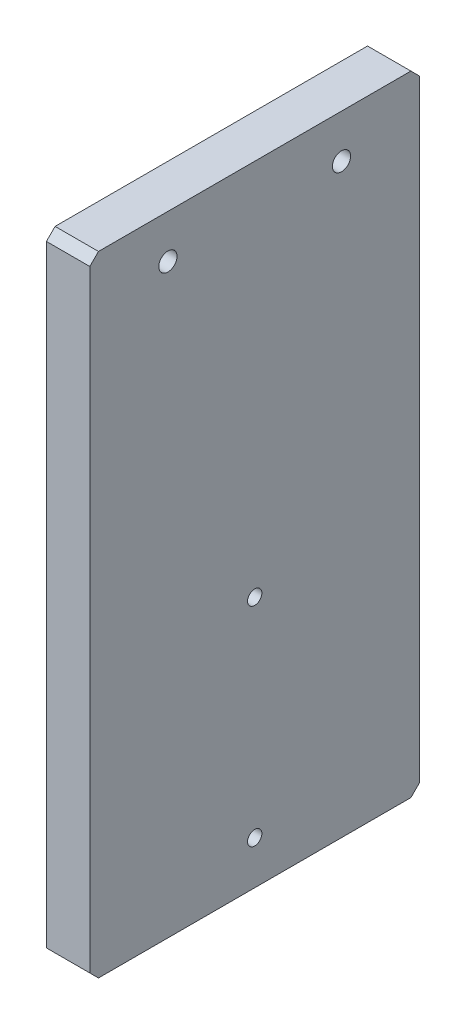
SolidWorks part; units mm, degrees
material "A6061"
ref_plane "前基準面" through (0, 0, 0) normal (0, 0, 1) x (1, 0, 0)
ref_plane "上基準面" through (0, 0, 0) normal (0, 1, 0) x (1, 0, 0)
ref_plane "右基準面" through (0, 0, 0) normal (1, 0, 0) x (0, 0, -1)
sketch "草图1" plane through (0, 0, 0) normal (1, 0, 0) x (0, 0, -1)
  line L1 (-38, 72.5) -> (38, 72.5)
  line L2 (-38, 72.5) -> (-38, -72.5)
  line L3 (-38, -72.5) -> (38, -72.5)
  line L4 (38, 72.5) -> (38, -72.5)
  line L5 (-38, 72.5) -> (38, -72.5) construction
  line L6 (-38, -72.5) -> (38, 72.5) construction
  point P0 (0, 0)
  dimension "D1" = 145
  dimension "D2" = 76
extrude "凸台-拉伸1" add sketch "草图1" along normal blind 10
sketch "草图2" plane through (10, 0, 0) normal (1, 0, 0) x (0, 0, -1)
  line L1 (38, 72.5) -> (-38, 72.5)
  line L2 (38, 72.5) -> (38, -22.5)
  line L3 (38, -22.5) -> (-38, -22.5)
  line L4 (-38, 72.5) -> (-38, -22.5)
  line L5 (-38, 72.5) -> (-38, -72.5) construction
  dimension "D1" = 95
  dimension "D2" = 76
sketch "草图7" plane through (0, 0, 0) normal (-1, 0, 0) x (0, 0, 1)
  line L1 (-38, 72.5) -> (38, 72.5) construction
  line L2 (0, 0) -> (0, 54.9907) construction
  point P0 (20, 62.5)
  point P2 (-20, 62.5)
  dimension "D1" = 40
  dimension "D3" = 10
hole_wizard "M5 螺纹孔1" positions "草图7" profile "草图8" tap size "M5" standard "GB" end condition through all
sketch "草图8" plane through (0, 62.5, 20) normal (0, 1, 0) x (0, 0, 1)
  line L0 (0, 0) -> (0, 10)
  line L1 (0, 10) -> (2.1, 10)
  line L2 (2.1, 10) -> (2.1, 0)
  line L5 (2.1, 0) -> (0, 0)
  line L11 (0, -6.35) -> (0, 107.95) construction
  dimension "通孔螺纹孔钻头直径" = 4.2
  dimension "通孔螺纹孔钻头深度" = 10
cosmetic thread "孔螺纹线1" parameters "D2"=5
cosmetic thread "孔螺纹线2" parameters "D2"=5
sketch "草图9" plane through (0, 0, 0) normal (-1, 0, 0) x (0, 0, 1)
  line L3 (38, -72.5) -> (-38, -72.5) construction
  line L5 (0, 0) -> (0, -67.3431) construction
  point P6 (0, -14.5)
  point P9 (0, -62.5)
  dimension "D3" = 48
  dimension "D4" = 10
hole_wizard "M4 螺纹孔1" positions "草图9" profile "草图10" tap size "M4" standard "GB" end condition through all
sketch "草图10" plane through (0, -14.5, 0) normal (0, 1, 0) x (0, 0, 1)
  line L0 (0, 0) -> (0, 10)
  line L1 (0, 10) -> (1.65, 10)
  line L2 (1.65, 10) -> (1.65, 0)
  line L5 (1.65, 0) -> (0, 0)
  line L11 (0, -6.35) -> (0, 107.95) construction
  dimension "通孔螺纹孔钻头直径" = 3.3
  dimension "通孔螺纹孔钻头深度" = 10
cosmetic thread "孔螺纹线3" parameters "D2"=4
cosmetic thread "孔螺纹线4" parameters "D2"=4
chamfer "倒角1" distance 2 angle 45 4 edges at (5, -72.5, 38) (5, 72.5, 38) (5, -72.5, -38) (5, 72.5, -38)
